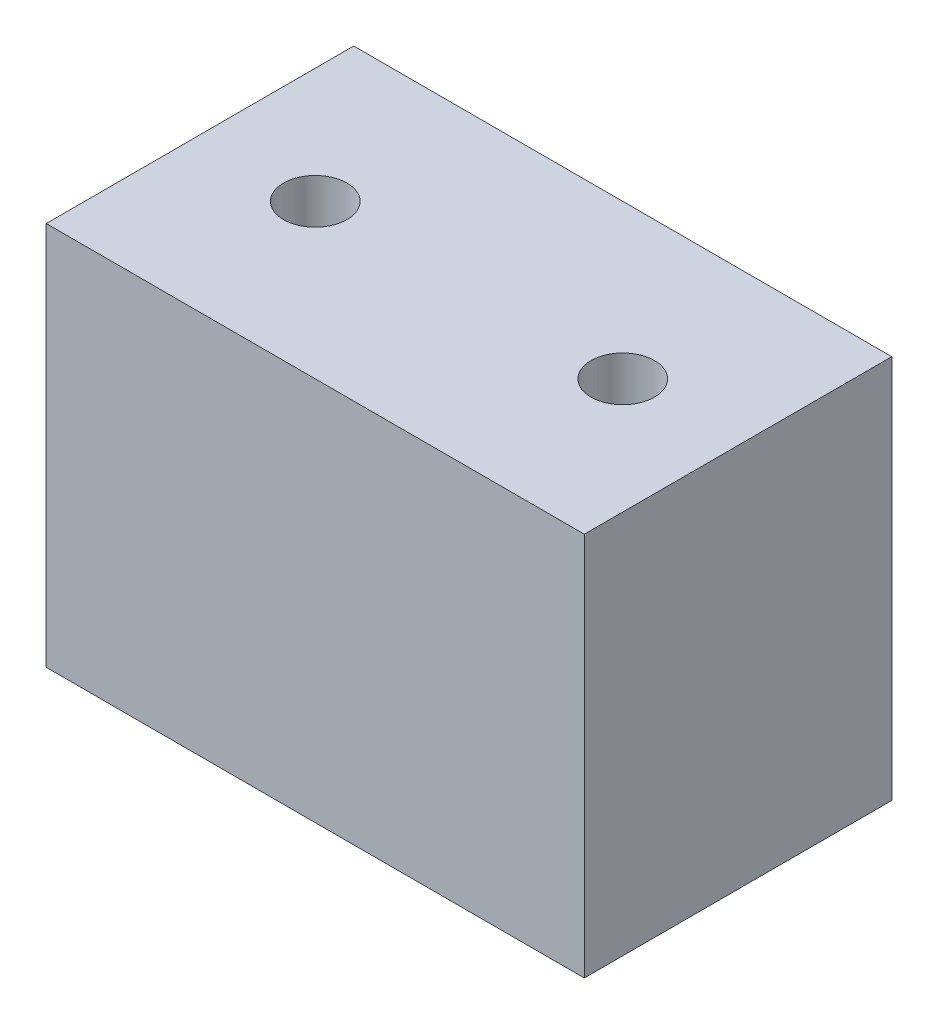
from build123d import *

# Parameters (mm, degrees)
SKETCH_1_W          = 28
SKETCH_1_H          = 20
EXTRUDE_1_DEPTH     = 8
SKETCH_2_R          = 1.65
CUT_EXTRUDE_1_DEPTH = 13


with BuildPart() as part:
    # 草图1 → 凸台-拉伸1 (new, symmetric)
    with BuildSketch(Plane.XY):
        Rectangle(SKETCH_1_W, SKETCH_1_H)
    extrude(amount=EXTRUDE_1_DEPTH, both=True)

    # 草图2 → 切除-拉伸1 (cut, symmetric)
    with BuildSketch(Plane(origin=(0, 0, 0), x_dir=(1, 0, 0), z_dir=(0, 1, 0))):
        with Locations(Location((-8, 0, 0), (0, 0, 270))):
            Circle(SKETCH_2_R)
        with Locations(Location((8, 0, 0), (0, 0, 270))):
            Circle(SKETCH_2_R)
    extrude(amount=CUT_EXTRUDE_1_DEPTH, both=True, mode=Mode.SUBTRACT)


solid = part.part
